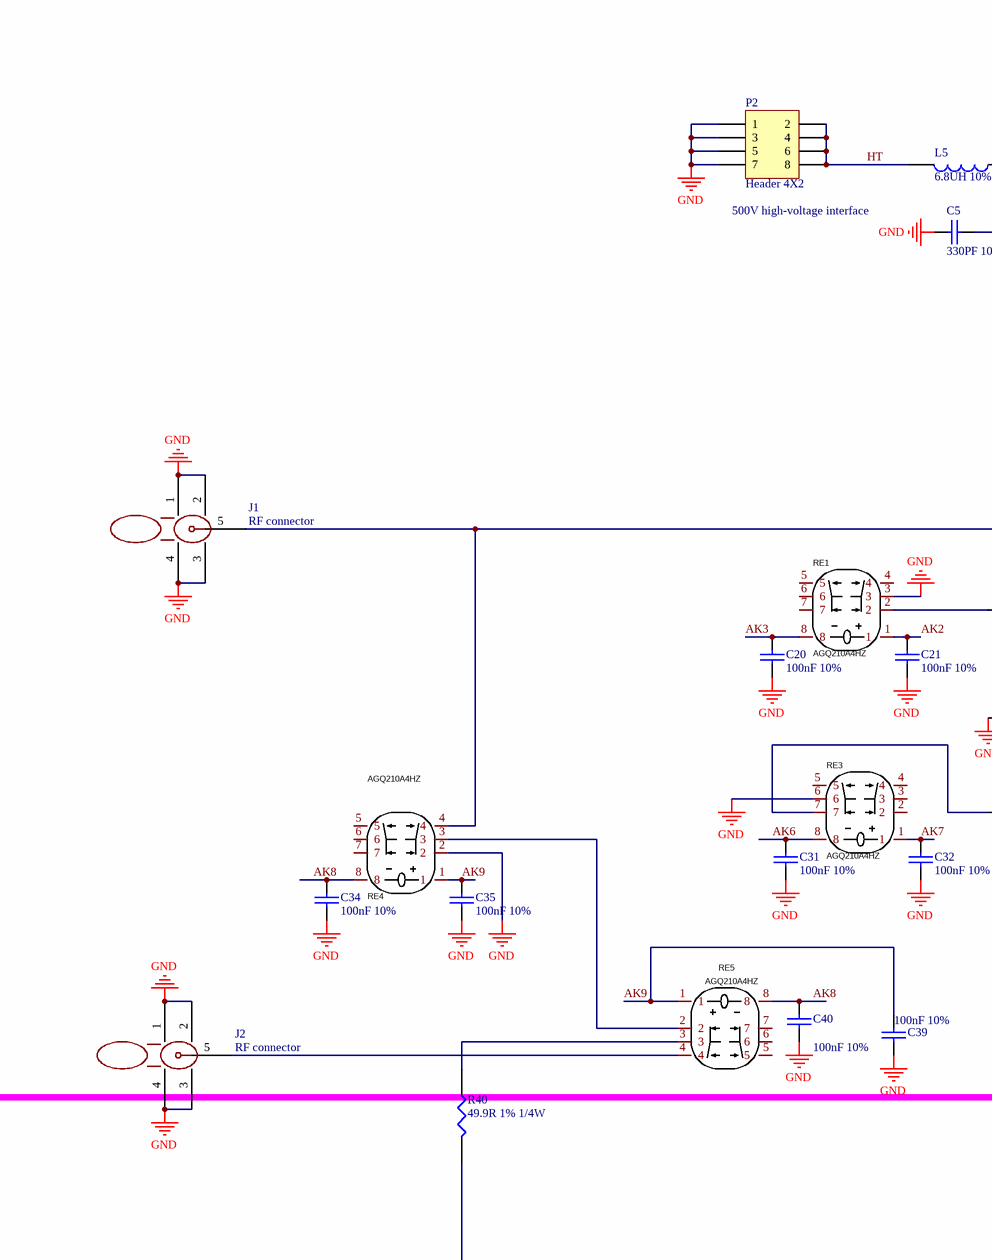
[diagram p0: PCBE109560-6.SchDoc, top left]
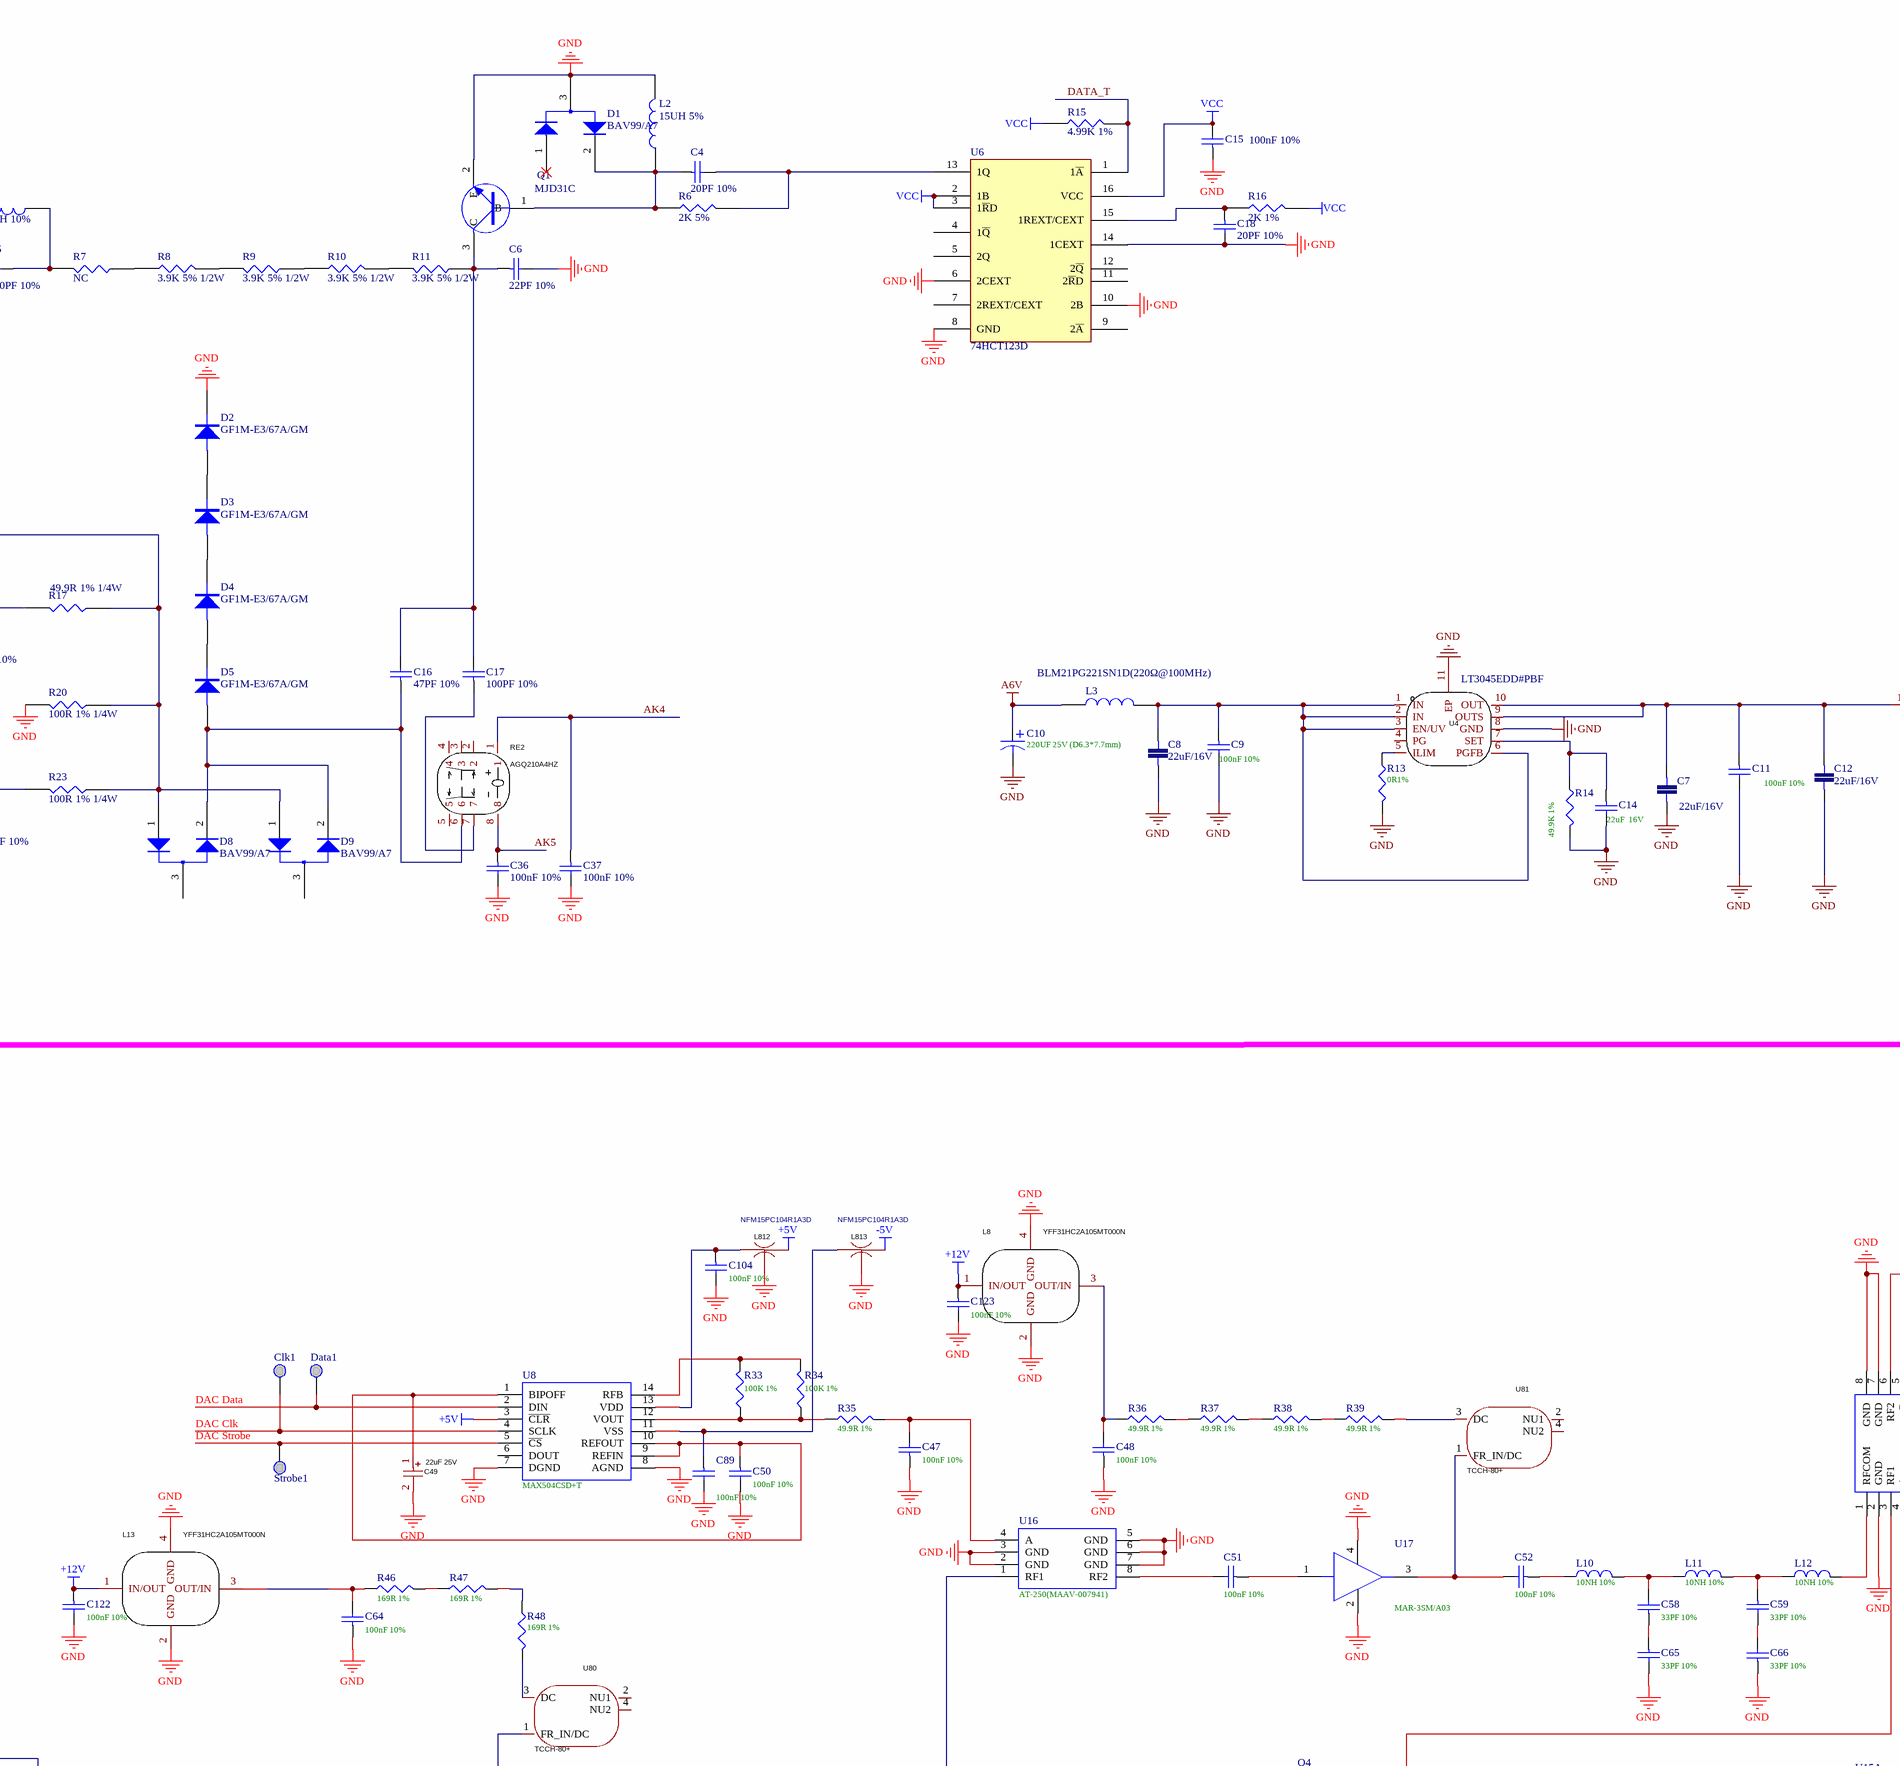
[diagram p1: PCBE109560-6.SchDoc, top middle]
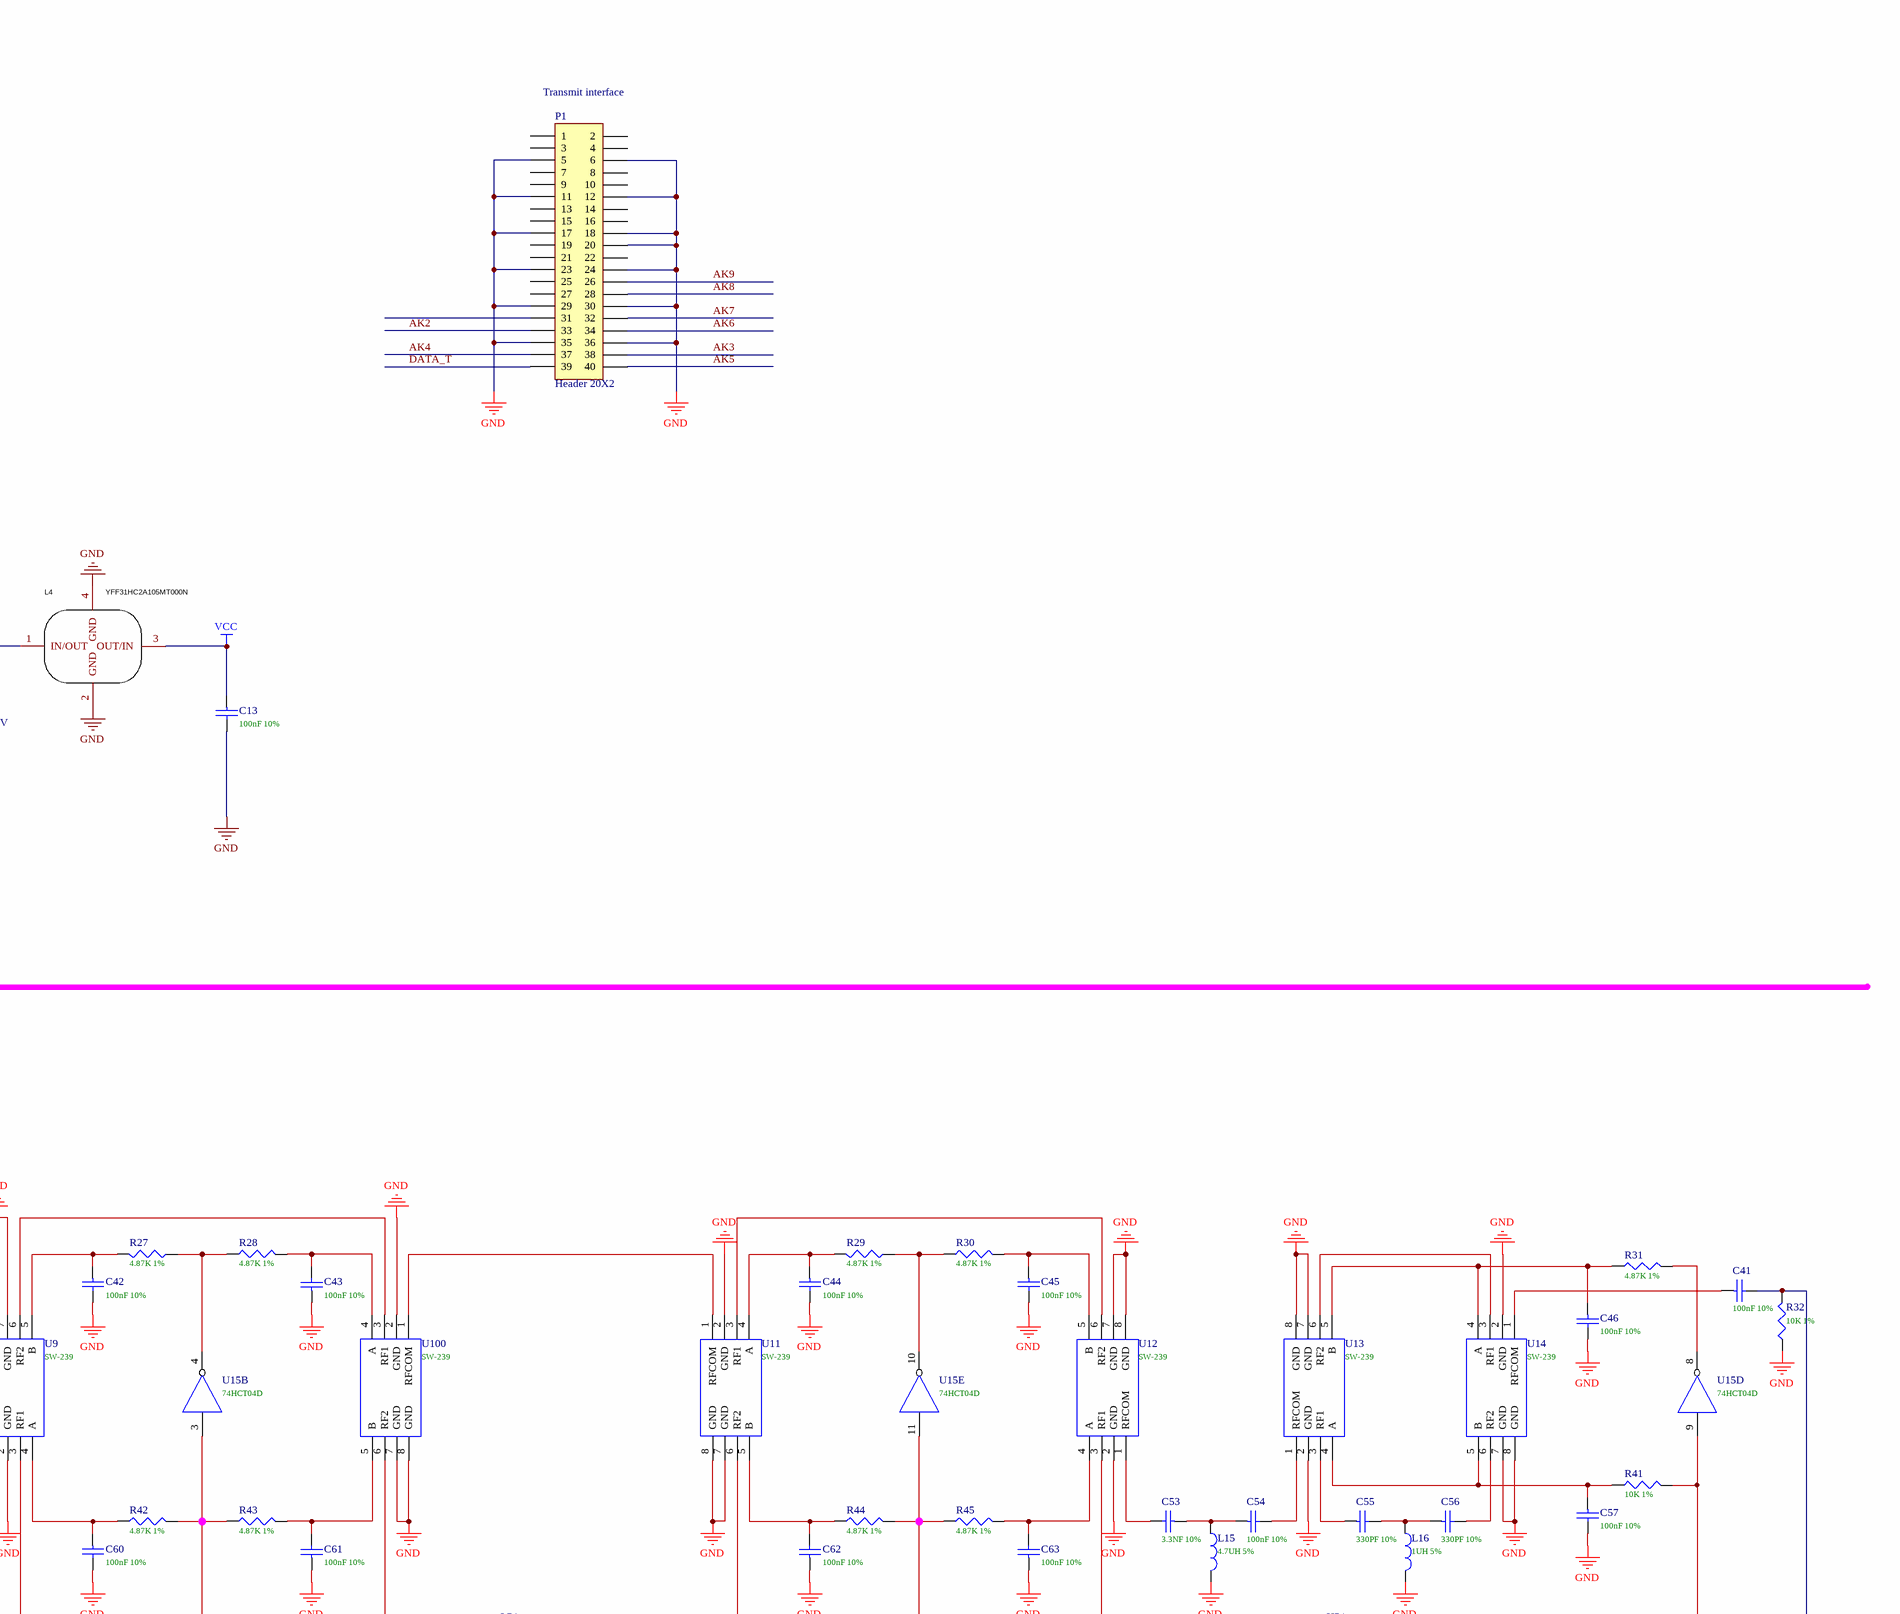
[diagram p2: PCBE109560-6.SchDoc, top right]
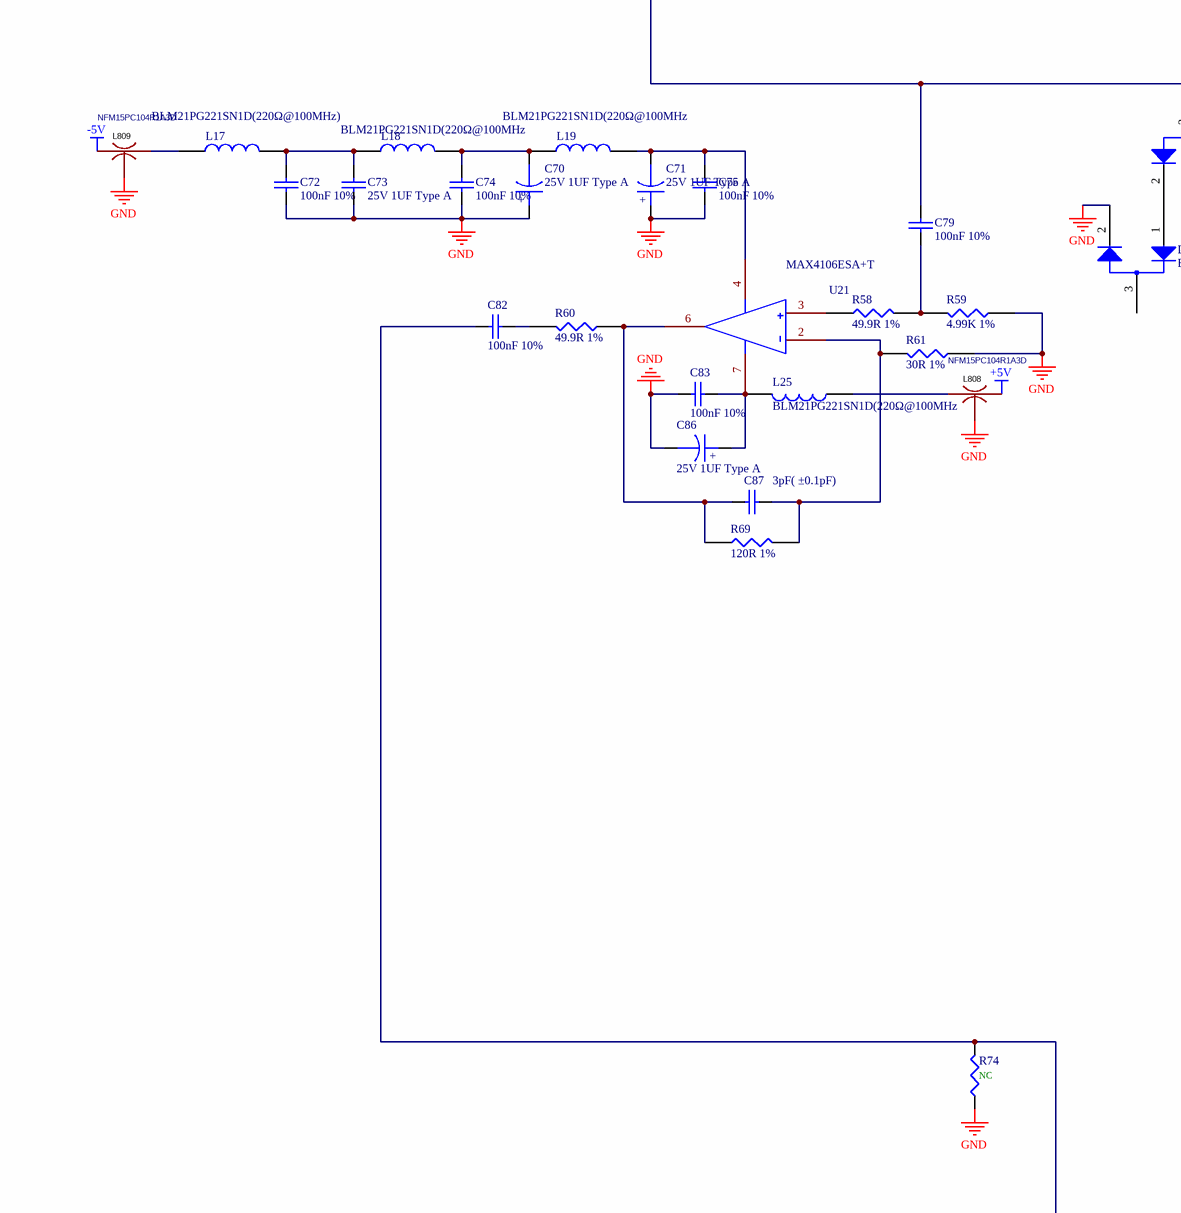
[diagram p3: PCBE109560-6.SchDoc, bottom left]
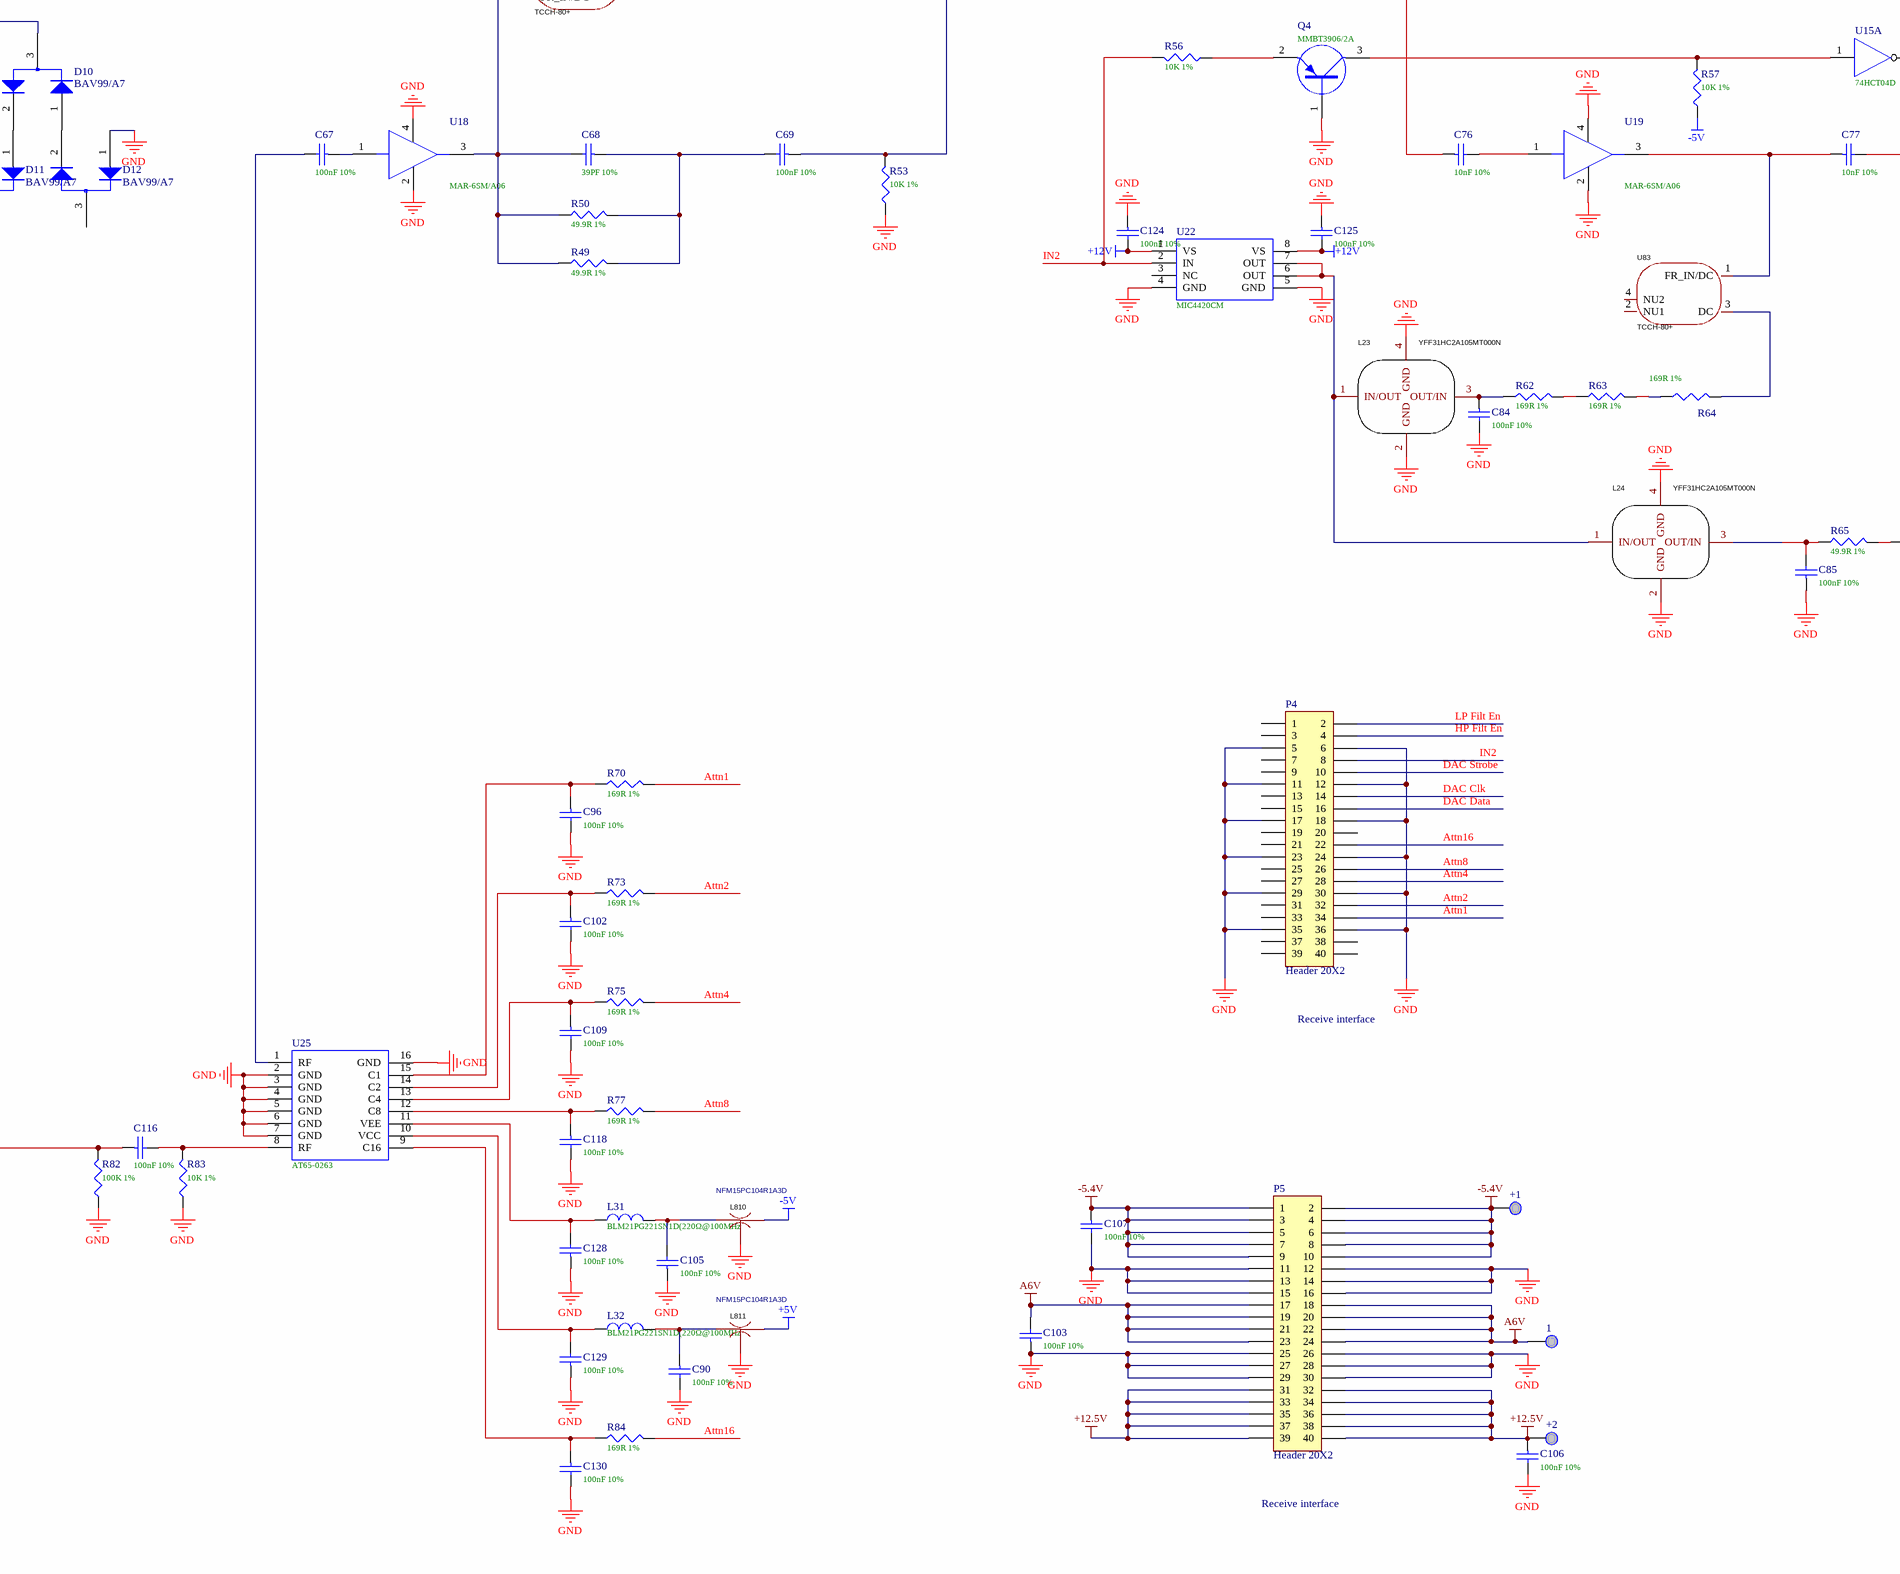
[diagram p4: PCBE109560-6.SchDoc, bottom middle]
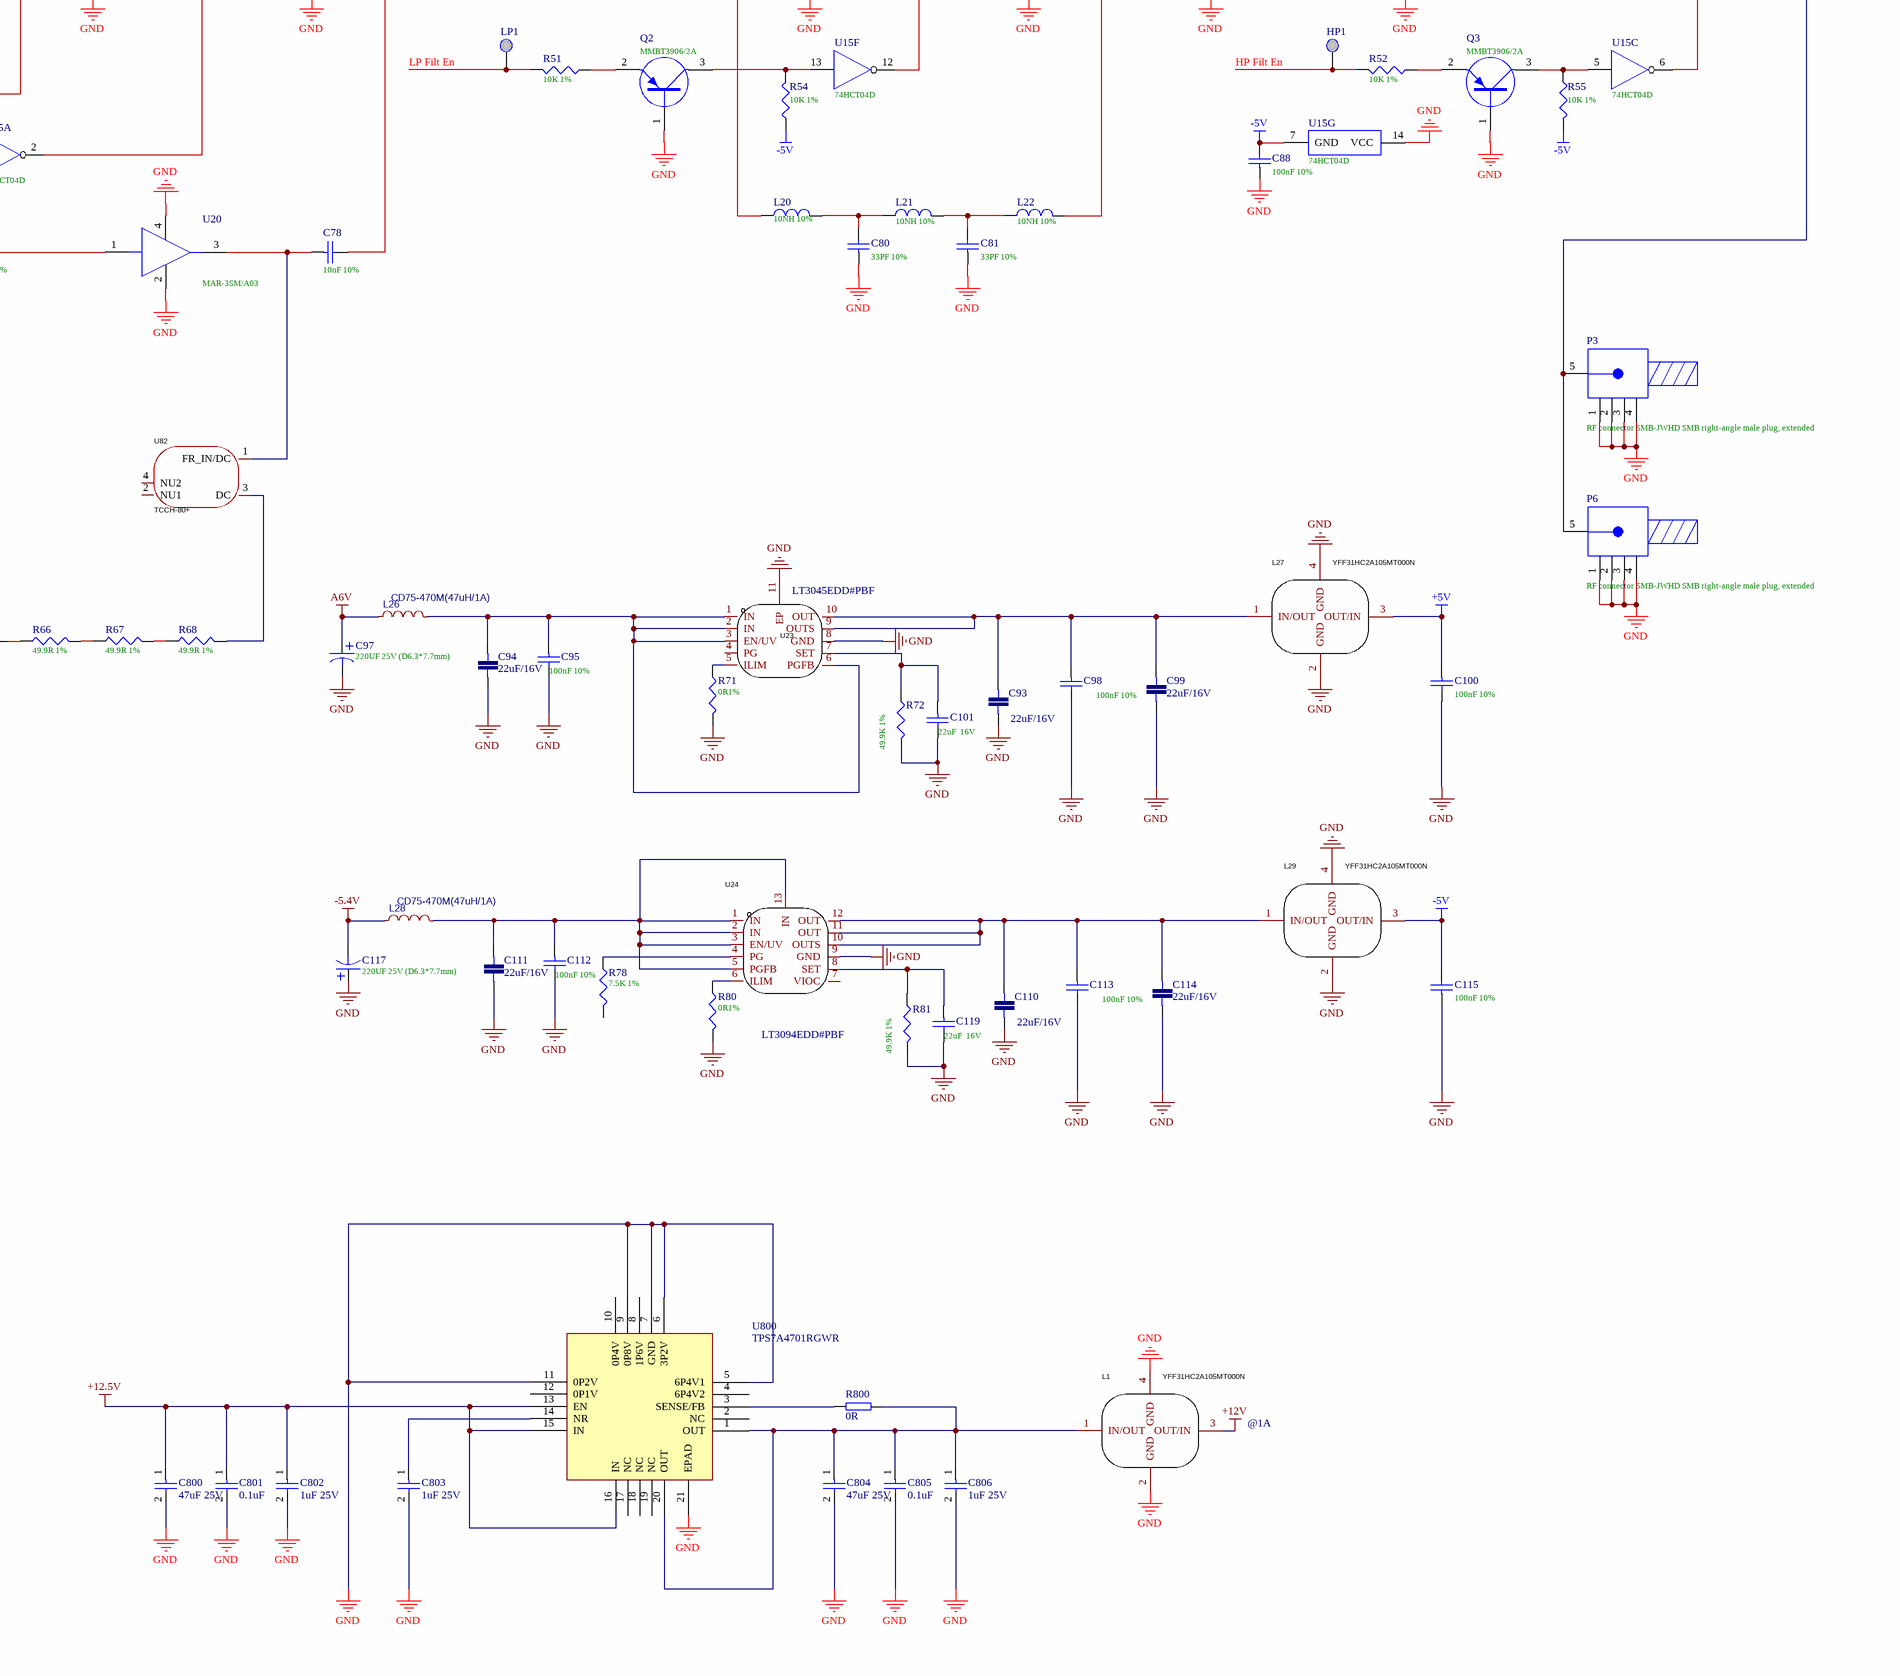
[diagram p5: PCBE109560-6.SchDoc, bottom right]
# Altium schematic sheet PCBE109560-6.SchDoc (part 1 of 2)
size E; SheetNumber: 0; SheetTotal: 0